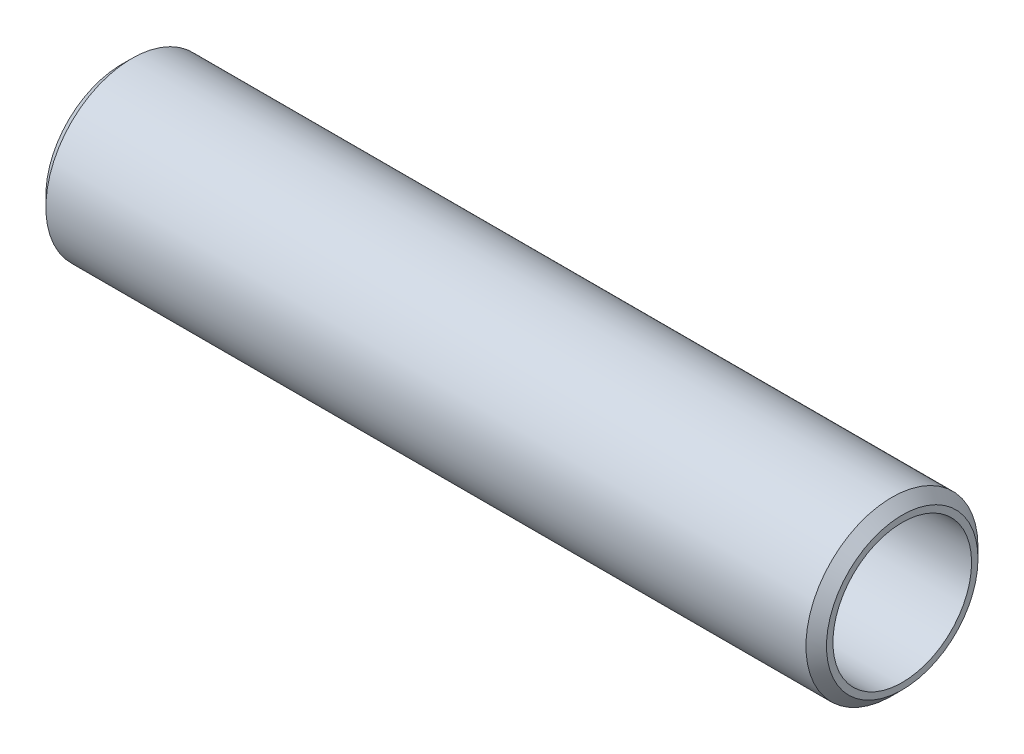
from build123d import *

# Parameters (mm, degrees)
SKETCH_1_R      = 16.75
SKETCH_1_R_2    = 13.5
EXTRUDE_1_DEPTH = 152
CHAMFER_1_SIZE  = 2


with BuildPart() as part:
    # 草图1 → 拉伸-薄壁1 (new body)
    with BuildSketch(Plane(origin=(0, 0, 0), x_dir=(0, 0, -1), z_dir=(1, 0, 0))):
        Circle(SKETCH_1_R)
        Circle(SKETCH_1_R_2, mode=Mode.SUBTRACT)
    extrude(amount=EXTRUDE_1_DEPTH)

    # 倒角1
    chamfer_1_edges = [part.edges().sort_by_distance(p)[0] for p in [
        (0, 0, 16.75),
        (152, 0, 16.75),
    ]]
    chamfer(chamfer_1_edges, length=CHAMFER_1_SIZE)


solid = part.part
